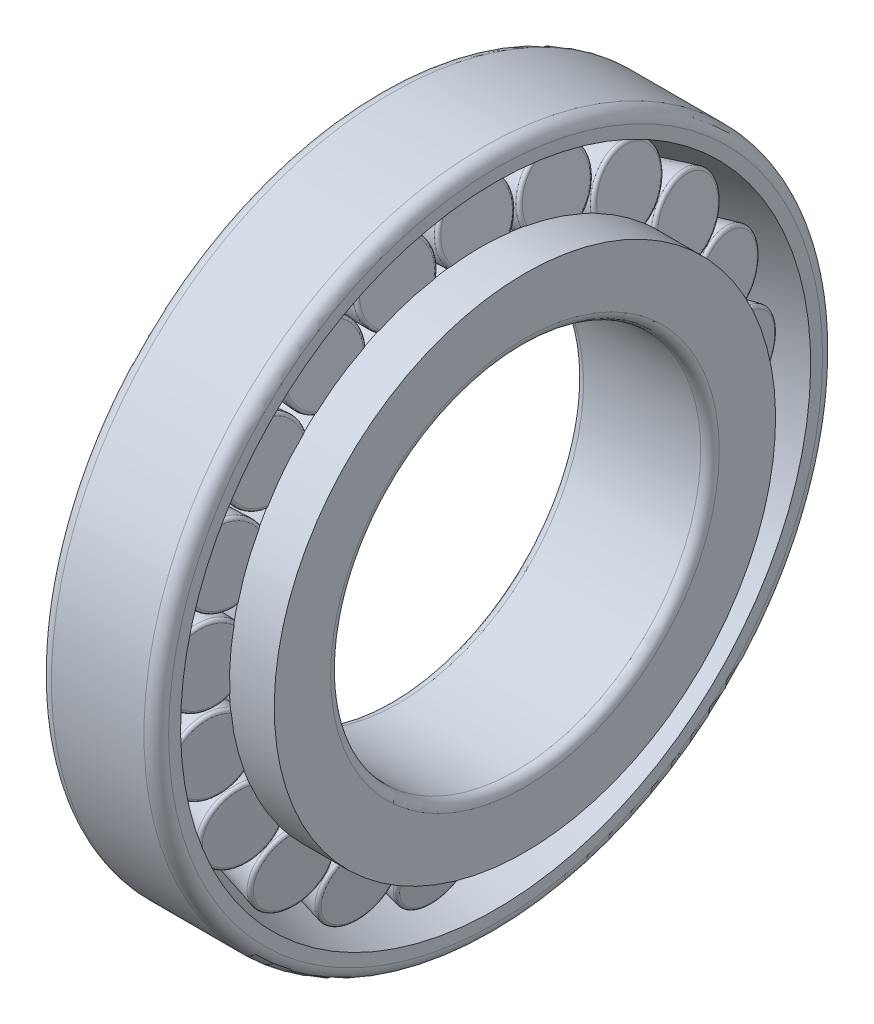
SolidWorks part; units mm, degrees
ref_plane "Front" through (0, 0, 0) normal (0, 0, 1) x (1, 0, 0)
ref_plane "Top" through (0, 0, 0) normal (0, 1, 0) x (1, 0, 0)
ref_plane "Right" through (0, 0, 0) normal (1, 0, 0) x (0, 0, -1)
sketch "Sketch1" plane through (0, 0, 0) normal (0, 0, 1) x (1, 0, 0)
  line L0 (14.25, 0) -> (13.9916, 0) construction
  line L1 (9.5, 51.0678) -> (9.5, 53)
  line L2 (7.5, 55) -> (-7.5, 55)
  line L3 (-9.5, 53) -> (-9.5, 45.938)
  line L4 (-9.5, 45.938) -> (9.5, 51.0678)
  line L5 (-7.75, 31.5) -> (-7.75, 38.0348)
  line L6 (-6.25, 30) -> (12.75, 30)
  line L7 (14.25, 31.5) -> (14.25, 40.6295)
  line L8 (-4.7446, 36.5348) -> (-6.5625, 46.7311)
  line L9 (7.5, 37.6295) -> (5.306, 49.9355)
  line L10 (-5.6536, 41.6329) -> (6.403, 43.7825) construction
  line L11 (-4.7446, 36.5348) -> (7.5, 37.6295)
  line L12 (6.9651, 42.5) -> (14.25, 42.5)
  line L13 (14.25, 40.6295) -> (6.9651, 40.6295)
  line L14 (-7.75, 38.0348) -> (-5.012, 38.0348)
  arc A0 (-7.5, 55) -> (-9.5, 53) centre (-7.5, 53) ccw
  arc A1 (9.5, 53) -> (7.5, 55) centre (7.5, 53) ccw
  arc A2 (-6.25, 30) -> (-7.75, 31.5) centre (-6.25, 31.5) cw
  arc A3 (12.75, 30) -> (14.25, 31.5) centre (12.75, 31.5) ccw
  point P19 (-9.5, 55)
  point P22 (9.5, 55)
  point P24 (0, 55)
  point P29 (-7.75, 30)
  point P32 (14.25, 30)
revolve "Revolve1" add sketch "Sketch1" angle 360 about L0
sketch "Sketch2" plane through (0, 0, 0) normal (0, 0, 1) x (1, 0, 0)
  line L0 (-5.6732, 41.6294) -> (5.8369, 43.6816) construction
  line L4 (-5.6536, 41.6329) -> (6.403, 43.7825) construction
  line L5 (-5.6732, 41.6294) -> (6.4227, 43.786)
  line L7 (-6.5822, 46.7276) -> (-4.7611, 36.5132)
  line L8 (7.5235, 37.6115) -> (5.3257, 49.939)
  line L9 (-4.7611, 36.5132) -> (7.5235, 37.6115)
  line L10 (-5.6732, 41.6294) -> (-4.8415, 36.9643)
  line L11 (7.4277, 38.1487) -> (6.4227, 43.786)
  line L12 (-4.3047, 36.554) -> (6.98, 37.5629)
  arc A0 (-4.3047, 36.554) -> (-4.8415, 36.9643) centre (-4.3493, 37.052) cw
  arc A1 (6.98, 37.5629) -> (7.4277, 38.1487) centre (6.9355, 38.061) ccw
revolve "Revolve2" add sketch "Sketch2" angle 360 about L0
sketch "Sketch3" plane through (0, 0, 0) normal (0, 0, 1) x (1, 0, 0)
  line L0 (-9.5, 45.938) -> (9.5, 51.0678) construction
  line L1 (-9.5, 53) -> (-9.5, 45.938) construction
  line L2 (7.5, 55) -> (-7.5, 55) construction
  line L3 (9.5, 51.0678) -> (9.5, 53) construction
  line L4 (-9.5, 45.938) -> (9.5, 51.0678)
  line L5 (-9.5, 53) -> (-9.5, 45.938)
  line L6 (7.5, 55) -> (-7.5, 55)
  line L7 (9.5, 51.0678) -> (9.5, 53)
  arc A0 (-7.5, 55) -> (-9.5, 53) centre (-7.5, 53) ccw construction
  arc A1 (9.5, 53) -> (7.5, 55) centre (7.5, 53) ccw construction
  arc A2 (-7.5, 55) -> (-9.5, 53) centre (-7.5, 53) ccw
  arc A3 (9.5, 53) -> (7.5, 55) centre (7.5, 53) ccw
revolve "Revolve3" add sketch "Sketch3" angle 360 about axis through (14.25, 0, 0) along (-1, 0, 0)
pattern_circular "Circular-Pattern1" count 21 over 360 about axis through (0, 0, 0) along (1, 0, 0) of "Revolve2"
equation "\"gzzj@Sketch1\" =  ( \"DD@Sketch1\" - \"XD@Sketch1\" )  / 4"
equation "\"D1@Sketch1\" = \"DB@Sketch1\" - \"DT@Sketch1\" / 20"
equation "\"D2@Sketch1\" = \"DT@Sketch1\" - \"DC@Sketch1\" + \"XR12@Sketch1\""
equation "\"D4@Sketch1\" = \"D3@Sketch1\" / 2"
equation "\"D2@Sketch2\" = \"gzzj@Sketch1\" / 25"
equation "\"ZJ@Sketch1\" =  ( \"DD@Sketch1\" + \"XD@Sketch1\" )  / 2"
equation "\"D1@Circular-Pattern1\" = int( 3.14159265 / atn(( \"gzzj@Sketch1\" / 2) / sqr( \"ZJ@Sketch1\" * \"ZJ@Sketch1\" /4 - ( \"gzzj@Sketch1\"/ 2) *  ( \"gzzj@Sketch1\"/ 2))))"
